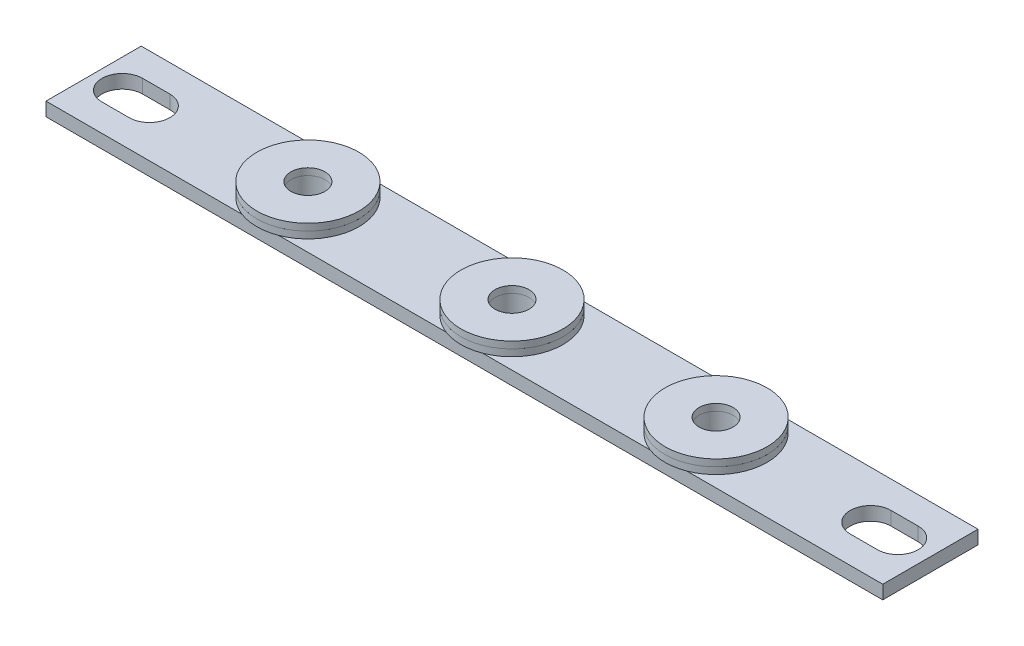
SolidWorks part; units mm, degrees
ref_plane "Front Plane" through (0, 0, 0) normal (0, 0, 1) x (1, 0, 0)
ref_plane "Top Plane" through (0, 0, 0) normal (0, 1, 0) x (1, 0, 0)
ref_plane "Right Plane" through (0, 0, 0) normal (1, 0, 0) x (0, 0, -1)
sketch "Sketch1" plane through (0, 0, 0) normal (0, 1, 0) x (1, 0, 0)
  line L0 (-57.2857, 0) -> (-53.2857, 0) construction
  line L1 (-61.5, -7) -> (61.5, -7)
  line L2 (-61.5, -7) -> (-61.5, 7)
  line L3 (-61.5, 7) -> (61.5, 7)
  line L4 (61.5, -7) -> (61.5, 7)
  line L5 (-61.5, -7) -> (61.5, 7) construction
  line L6 (-61.5, 7) -> (61.5, -7) construction
  line L7 (-57.2857, 3) -> (-53.2857, 3)
  line L8 (-57.2857, -3) -> (-53.2857, -3)
  line L9 (52.7143, 0) -> (56.7143, 0) construction
  line L10 (52.7143, 3) -> (56.7143, 3)
  line L11 (52.7143, -3) -> (56.7143, -3)
  arc A0 (-57.2857, 3) -> (-57.2857, -3) centre (-57.2857, 0) ccw
  arc A1 (-53.2857, -3) -> (-53.2857, 3) centre (-53.2857, 0) ccw
  arc A2 (52.7143, 3) -> (52.7143, -3) centre (52.7143, 0) ccw
  arc A3 (56.7143, -3) -> (56.7143, 3) centre (56.7143, 0) ccw
  circle A4 centre (-30, 0) radius 2.5
  circle A5 centre (0, 0) radius 2.5
  circle A6 centre (30, 0) radius 2.5
  point P0 (0, 0)
  point P8 (-55.2857, 0)
  point P13 (54.7143, 0)
  dimension "D4" = 3
  dimension "D5" = 3
  dimension "D8" = 5
  dimension "D9" = 5
  dimension "D10" = 5
  dimension "D1" = 123
  dimension "D2" = 14
  dimension "D3" = 110
  dimension "D6" = 4
  dimension "D7" = 4
  dimension "D11" = 30
  dimension "D12" = 30
extrude "Boss-Extrude1" add sketch "Sketch1" along normal blind 2
sketch "Sketch2" plane through (0, 2, 0) normal (0, 1, 0) x (1, 0, 0)
  circle A0 centre (-30, 0) radius 2.5
  circle A1 centre (-30, 0) radius 7.5
  circle A2 centre (0, 0) radius 7.5
  circle A3 centre (0, 0) radius 2.5
  circle A4 centre (30, 0) radius 2.5
  circle A5 centre (30, 0) radius 7.5
  dimension "D1" = 15
  dimension "D2" = 15
  dimension "D3" = 15
extrude "Boss-Extrude2" add sketch "Sketch2" along normal blind 1
sketch "Sketch3" plane through (0, 3, 0) normal (0, 1, 0) x (1, 0, 0)
  circle A0 centre (-30, 0) radius 2.5
  circle A1 centre (-30, 0) radius 7.5
  circle A2 centre (-30, 0) radius 7.5
  circle A3 centre (0, 0) radius 7.5
  circle A4 centre (0, 0) radius 2.5
  circle A5 centre (30, 0) radius 2.5
  circle A6 centre (30, 0) radius 7.5
  dimension "D2" = 15
  dimension "D3" = 15
  dimension "D1" = 0
extrude "Boss-Extrude3" add sketch "Sketch3" along normal blind 1 separate body
